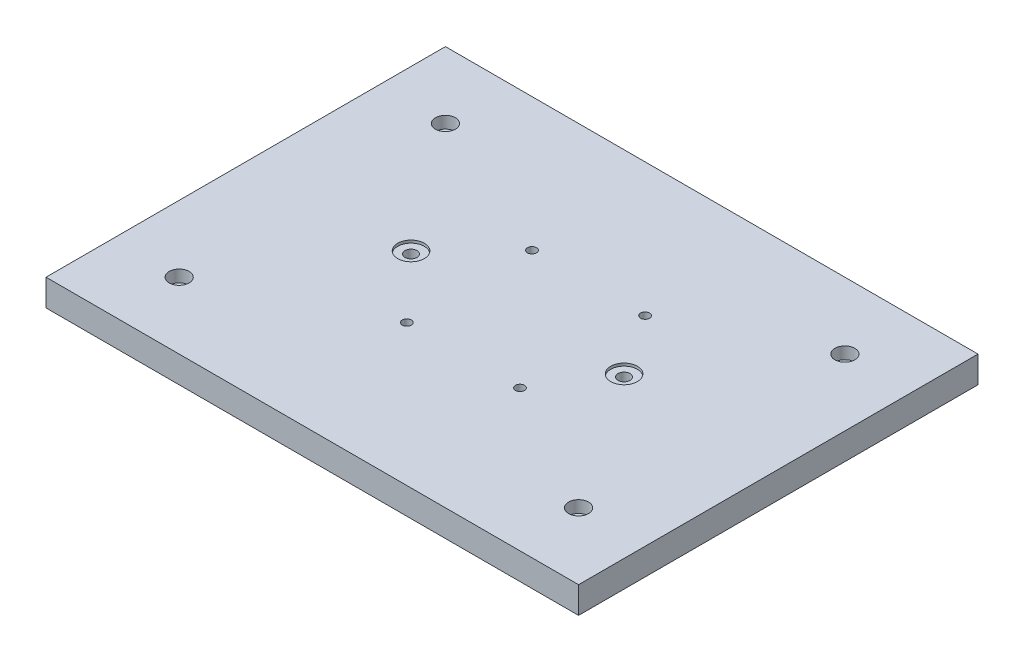
from build123d import *

# Parameters (mm, degrees)
SKETCH1_W                                            = 400
SKETCH1_H                                            = 300
BOSS_EXTRUDE1_DEPTH                                  = 20
HOLE_SIZE_PER_SOCKET_HEAD_CAP_SCREW_TYPE_D           = 9
HOLE_SIZE_PER_SOCKET_HEAD_CAP_SCREW_TYPE_CBORE_D     = 15
HOLE_SIZE_PER_SOCKET_HEAD_CAP_SCREW_TYPE_CBORE_DEPTH = 9
SKETCH5_R                                            = 10
CUT_EXTRUDE1_DEPTH                                   = 2
HOLE_SIZE_PER_SOCKET_HEAD_CAP_SCREW_2_D              = 9
HOLE_SIZE_PER_SOCKET_HEAD_CAP_SCREW_2_CBORE_D        = 15
HOLE_SIZE_PER_SOCKET_HEAD_CAP_SCREW_2_CBORE_DEPTH    = 9
M8_TAPPED_HOLE1_D                                    = 6.8


with BuildPart() as part:
    # Sketch1 → Boss-Extrude1 (new body)
    with BuildSketch(Plane(origin=(0, 0, 0), x_dir=(1, 0, 0), z_dir=(0, 1, 0))):
        Rectangle(SKETCH1_W, SKETCH1_H)
    extrude(amount=BOSS_EXTRUDE1_DEPTH)

    # Hole size per socket head cap screw type (through all)
    with Locations(Plane(origin=(0, 20, 0), x_dir=(1, 0, 0), z_dir=(0, 1, 0))):
        with Locations((-150, 100), (-150, -100), (150, 100), (150, -100)):
            CounterBoreHole(HOLE_SIZE_PER_SOCKET_HEAD_CAP_SCREW_TYPE_D / 2, HOLE_SIZE_PER_SOCKET_HEAD_CAP_SCREW_TYPE_CBORE_D / 2, HOLE_SIZE_PER_SOCKET_HEAD_CAP_SCREW_TYPE_CBORE_DEPTH)

    # Sketch5 → Cut-Extrude1 (cut)
    with BuildSketch(Plane(origin=(0, 20, 0), x_dir=(1, 0, 0), z_dir=(0, 1, 0))):
        with Locations(Location((-80, 4.166410727, 0), (0, 0, 270))):
            Circle(SKETCH5_R)
        with Locations(Location((80, 4.166410727, 0), (0, 0, 270))):
            Circle(SKETCH5_R)
    extrude(amount=-CUT_EXTRUDE1_DEPTH, mode=Mode.SUBTRACT)

    # Hole size per socket head cap screw  2 (through all)
    with Locations(Plane(origin=(0, 0, 0), x_dir=(-1, 0, 0), z_dir=(0, -1, 0))):
        with Locations((80, 4.166410727), (-80, 4.166410727)):
            CounterBoreHole(HOLE_SIZE_PER_SOCKET_HEAD_CAP_SCREW_2_D / 2, HOLE_SIZE_PER_SOCKET_HEAD_CAP_SCREW_2_CBORE_D / 2, HOLE_SIZE_PER_SOCKET_HEAD_CAP_SCREW_2_CBORE_DEPTH)

    # M8 Tapped Hole1 (through all)
    with Locations(Plane(origin=(0, 20, 0), x_dir=(1, 0, 0), z_dir=(0, 1, 0))):
        with Locations((-35, 50), (-35, -44), (50, -44), (50, 50)):
            Hole(M8_TAPPED_HOLE1_D / 2)


solid = part.part
